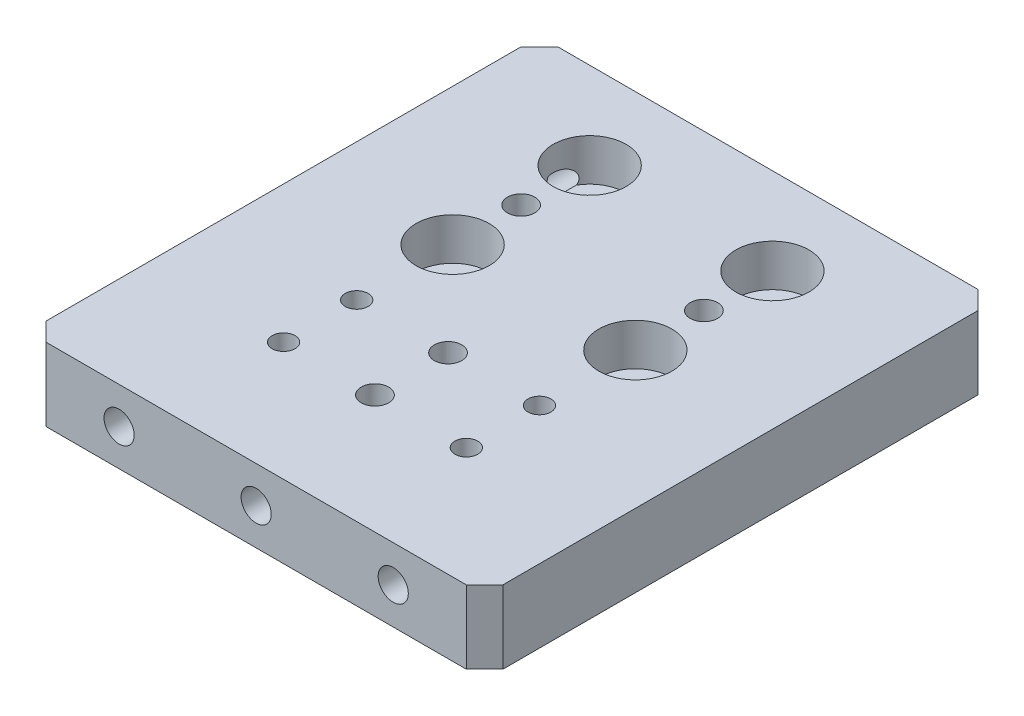
from build123d import *

# Parameters (mm, degrees)
SKETCH_1_W                = 50
SKETCH_1_H                = 56
EXTRUDE_1_DEPTH           = 8
HOLE_WIZARD_M4_1_D        = 3.3
HOLE_WIZARD_M4_1_DEPTH    = 10.1
HOLE_WIZARD_M4_1_TIP      = 0.991420021
CHAMFER_1_SIZE            = 2
HOLE_WIZARD_M4_2_D        = 3.3
HOLE_WIZARD_M4_2_DEPTH    = 10.1
HOLE_WIZARD_M4_2_TIP      = 0.991420021
MM_1_D                    = 3
MM_1_DEPTH                = 12.4
MM_1_TIP                  = 0.901290929
HOLE_WIZARD_M3_1_D        = 2.5
HOLE_WIZARD_M3_1_DEPTH    = 15
HOLE_WIZARD_M3_1_TIP      = 0.751075774
MM_2_D                    = 3
MM_2_DEPTH                = 15
MM_2_TIP                  = 0.901290929
HOLE_WIZARD_1_D           = 4.5
HOLE_WIZARD_1_DEPTH       = 15
HOLE_WIZARD_1_CBORE_D     = 8
HOLE_WIZARD_1_CBORE_DEPTH = 4.6
HOLE_WIZARD_1_TIP         = 1.351936393
HOLE_WIZARD_2_D           = 4.5
HOLE_WIZARD_2_DEPTH       = 15
HOLE_WIZARD_2_CBORE_D     = 8
HOLE_WIZARD_2_CBORE_DEPTH = 4.6
HOLE_WIZARD_2_TIP         = 1.351936393
MM_3_D                    = 3
MM_3_DEPTH                = 15
MM_3_TIP                  = 0.901290929
CHAMFER_2_SIZE            = 2


with BuildPart() as part:
    # 草图1 → 凸台-拉伸1 (new body)
    with BuildSketch(Plane(origin=(0, 0, 0), x_dir=(1, 0, 0), z_dir=(0, 1, 0))):
        Rectangle(SKETCH_1_W, SKETCH_1_H)
    extrude(amount=EXTRUDE_1_DEPTH)

    # M4 螺纹孔1
    with Locations(Plane.XY.offset(28)):
        with Locations((15, 4), (0, 4), (-15, 4)):
            Hole(HOLE_WIZARD_M4_1_D / 2, depth=HOLE_WIZARD_M4_1_DEPTH)
            with Locations((0, 0, -(HOLE_WIZARD_M4_1_DEPTH + HOLE_WIZARD_M4_1_TIP / 2))):  # 118° drill point
                Cone(0, HOLE_WIZARD_M4_1_D / 2, HOLE_WIZARD_M4_1_TIP, mode=Mode.SUBTRACT)

    # 倒角1
    chamfer_1_edges = [part.edges().sort_by_distance(p)[0] for p in [
        (25, 4, 28),
        (-25, 4, 28),
    ]]
    chamfer(chamfer_1_edges, length=CHAMFER_1_SIZE)

    # M4 螺纹孔2
    with Locations(Plane(origin=(0, 0, -28), x_dir=(-1, 0, 0), z_dir=(0, 0, -1))):
        with Locations((-15, 4), (0, 4), (15, 4)):
            Hole(HOLE_WIZARD_M4_2_D / 2, depth=HOLE_WIZARD_M4_2_DEPTH)
            with Locations((0, 0, -(HOLE_WIZARD_M4_2_DEPTH + HOLE_WIZARD_M4_2_TIP / 2))):  # 118° drill point
                Cone(0, HOLE_WIZARD_M4_2_D / 2, HOLE_WIZARD_M4_2_TIP, mode=Mode.SUBTRACT)

    # 大小mm 暗销孔1
    with Locations(Plane(origin=(0, 0, 0), x_dir=(-1, 0, 0), z_dir=(0, -1, 0))):
        with Locations((0, -7), (0, -15)):
            Hole(MM_1_D / 2, depth=MM_1_DEPTH)
            with Locations((0, 0, -(MM_1_DEPTH + MM_1_TIP / 2))):  # 118° drill point
                Cone(0, MM_1_D / 2, MM_1_TIP, mode=Mode.SUBTRACT)

    # M3 螺纹孔1
    with Locations(Plane(origin=(0, 0, 0), x_dir=(-1, 0, 0), z_dir=(0, -1, 0))):
        with Locations((-10, -7), (10, -7), (-10, -15), (10, -15)):
            Hole(HOLE_WIZARD_M3_1_D / 2, depth=HOLE_WIZARD_M3_1_DEPTH)
            with Locations((0, 0, -(HOLE_WIZARD_M3_1_DEPTH + HOLE_WIZARD_M3_1_TIP / 2))):  # 118° drill point
                Cone(0, HOLE_WIZARD_M3_1_D / 2, HOLE_WIZARD_M3_1_TIP, mode=Mode.SUBTRACT)

    # 大小mm 暗销孔2
    with Locations(Plane(origin=(0, 8, 0), x_dir=(1, 0, 0), z_dir=(0, 1, 0))):
        with Locations((-10, 11)):
            Hole(MM_2_D / 2, depth=MM_2_DEPTH)
            with Locations((0, 0, -(MM_2_DEPTH + MM_2_TIP / 2))):  # 118° drill point
                Cone(0, MM_2_D / 2, MM_2_TIP, mode=Mode.SUBTRACT)

    # 打孔尺寸(%根据)内六角圆柱头螺钉的类型1
    with Locations(Plane(origin=(0, 8, 0), x_dir=(1, 0, 0), z_dir=(0, 1, 0))):
        with Locations((-10, 18.5), (-10, 3.5)):
            CounterBoreHole(HOLE_WIZARD_1_D / 2, HOLE_WIZARD_1_CBORE_D / 2, HOLE_WIZARD_1_CBORE_DEPTH, depth=HOLE_WIZARD_1_DEPTH)
            with Locations((0, 0, -(HOLE_WIZARD_1_DEPTH + HOLE_WIZARD_1_TIP / 2))):  # 118° drill point
                Cone(0, HOLE_WIZARD_1_D / 2, HOLE_WIZARD_1_TIP, mode=Mode.SUBTRACT)

    # 打孔尺寸(%根据)内六角圆柱头螺钉的类型2
    with Locations(Plane(origin=(0, 8, 0), x_dir=(1, 0, 0), z_dir=(0, 1, 0))):
        with Locations((10, 18.5), (10, 3.5)):
            CounterBoreHole(HOLE_WIZARD_2_D / 2, HOLE_WIZARD_2_CBORE_D / 2, HOLE_WIZARD_2_CBORE_DEPTH, depth=HOLE_WIZARD_2_DEPTH)
            with Locations((0, 0, -(HOLE_WIZARD_2_DEPTH + HOLE_WIZARD_2_TIP / 2))):  # 118° drill point
                Cone(0, HOLE_WIZARD_2_D / 2, HOLE_WIZARD_2_TIP, mode=Mode.SUBTRACT)

    # 大小mm 暗销孔3
    with Locations(Plane(origin=(0, 8, 0), x_dir=(1, 0, 0), z_dir=(0, 1, 0))):
        with Locations((10, 11)):
            Hole(MM_3_D / 2, depth=MM_3_DEPTH)
            with Locations((0, 0, -(MM_3_DEPTH + MM_3_TIP / 2))):  # 118° drill point
                Cone(0, MM_3_D / 2, MM_3_TIP, mode=Mode.SUBTRACT)

    # 倒角2
    chamfer_2_edges = [part.edges().sort_by_distance(p)[0] for p in [
        (-25, 4, -28),
        (25, 4, -28),
    ]]
    chamfer(chamfer_2_edges, length=CHAMFER_2_SIZE)


solid = part.part
